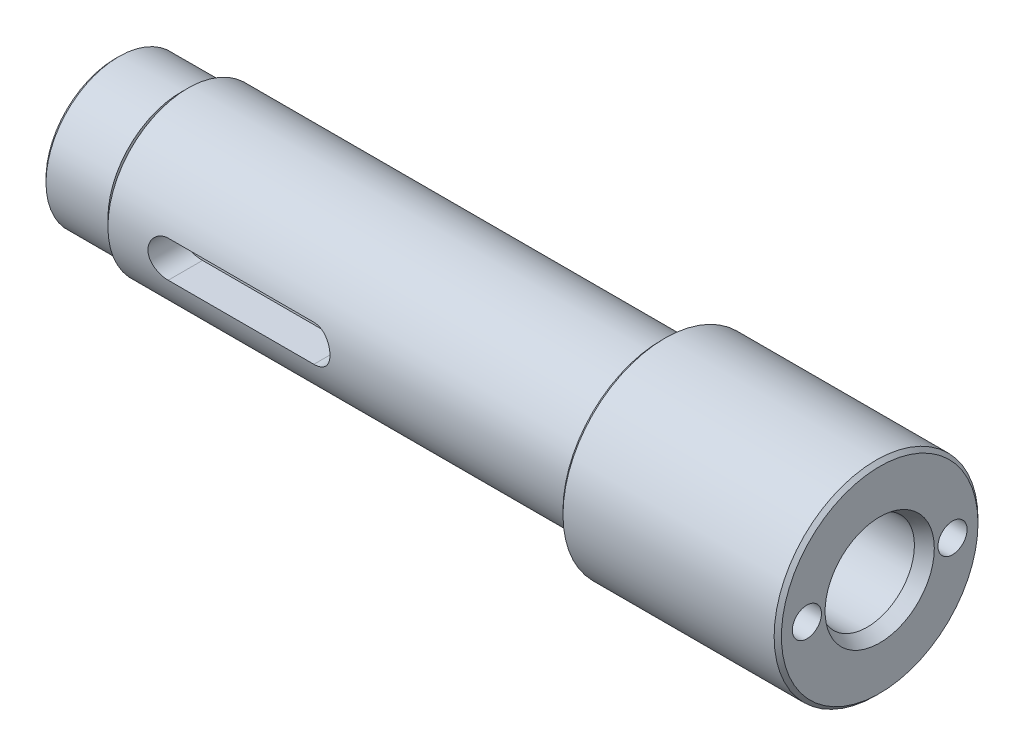
SolidWorks part; units mm, degrees
ref_plane "前视基准面" through (0, 0, 0) normal (0, 0, 1) x (1, 0, 0)
ref_plane "上视基准面" through (0, 0, 0) normal (0, 1, 0) x (1, 0, 0)
ref_plane "右视基准面" through (0, 0, 0) normal (1, 0, 0) x (0, 0, -1)
sketch "草图1" plane through (0, 0, 0) normal (1, 0, 0) x (0, 0, -1)
  circle A0 centre (0, 0) radius 14
  circle A1 centre (0, 0) radius 6.5
  dimension "D1" = 13
  dimension "D2" = 28
extrude "凸台-拉伸1" add sketch "草图1" along normal blind 105
sketch "草图2" plane through (0, 0, 0) normal (-1, 0, 0) x (0, 0, 1)
  circle A0 centre (0, 0) radius 14 construction
  circle A1 centre (0, 0) radius 14
  circle A2 centre (0, 0) radius 11
  dimension "D1" = 3
extrude "切除-拉伸1" cut sketch "草图2" against normal blind 75
sketch "草图3" plane through (0, 0, 0) normal (0, 1, 0) x (1, 0, 0)
  line L0 (-15.1033, 0) -> (6.2352, 0) construction
  line L1 (0, 16.2481) -> (0, 0)
  line L3 (0, 0) -> (4, 0)
  arc A0 (4, 0) -> (0, 16.2481) centre (-31, 0) ccw
  dimension "D1" = 4
  dimension "D2" = 35
sketch "草图4" plane through (0, 0, 0) normal (0, 0, 1) x (1, 0, 0)
  line L0 (18, 0) -> (38, 0) construction
  line L1 (18, 2.5) -> (38, 2.5)
  line L2 (18, -2.5) -> (38, -2.5)
  line L4 (0, 11) -> (0, -11) construction
  arc A0 (18, 2.5) -> (18, -2.5) centre (18, 0) ccw
  arc A1 (38, -2.5) -> (38, 2.5) centre (38, 0) ccw
  point P3 (28, 0)
  dimension "D1" = 2.5
  dimension "D2" = 20
  dimension "D3" = 18
extrude "切除-拉伸2" cut sketch "草图4" against normal mid plane 50
sketch "草图7" plane through (0, 0, 0) normal (-1, 0, 0) x (0, 0, 1)
  circle A0 centre (0, 0) radius 10
  circle A1 centre (0, 0) radius 11 construction
  circle A2 centre (0, 0) radius 11
  dimension "D1" = 20
extrude "切除-拉伸3" cut sketch "草图7" against normal blind 10
cosmetic thread "装饰螺纹线2" parameters "D1"=9, "D2"=17.294
sketch "草图8" plane through (0, 0, 0) normal (0, 0, 1) x (1, 0, 0)
  line L0 (0, 0) -> (4.0537, 0) construction
  line L1 (10, 10) -> (9, 10)
  line L2 (10, 10) -> (10, 8.5)
  line L3 (10, 8.5) -> (9, 8.5)
  line L4 (9, 10) -> (9, 8.5)
  dimension "D1" = 1
  dimension "D2" = 1.5
revolve "切除-旋转2" cut sketch "草图8" angle 360 about L0
chamfer "倒角1" distance 0.5 angle 45 3 edges at (75, 0, 14) (105, 0, -14) (0, 0, 10)
ref_plane "基准面1" through (0, 0, 0) normal (0, 1, 0) x (1, 0, 0)
hole_wizard "Ø4.0 (4) 直径孔1" positions "草图10" profile "草图9" hole size "Ø4.0" standard "GB"
sketch "草图10" plane through (105, 0, 0) normal (1, 0, 0) x (0, 0, -1)
  point P0 (-10, 0)
  point P2 (10, 0)
  dimension "D1" = 20
  dimension "D2" = 10
sketch "草图9" plane through (105, 0, 10) normal (0, 1, 0) x (0, 0, -1)
  line L0 (0, 0) -> (0, 9.2017)
  line L1 (0, 9.2017) -> (2, 8)
  line L2 (2, 8) -> (2, 0)
  line L5 (2, 0) -> (0, 0)
  line L10 (0, 9.2017) -> (-2, 8) construction
  line L11 (0, -6.35) -> (0, 107.95) construction
  dimension "孔直径" = 4
  dimension "孔深度" = 8
  dimension "导头角度" = 118
chamfer "倒角2" distance 1 angle 60 2 edges at (105, 0, -6.5) (0, 0, -6.5)
